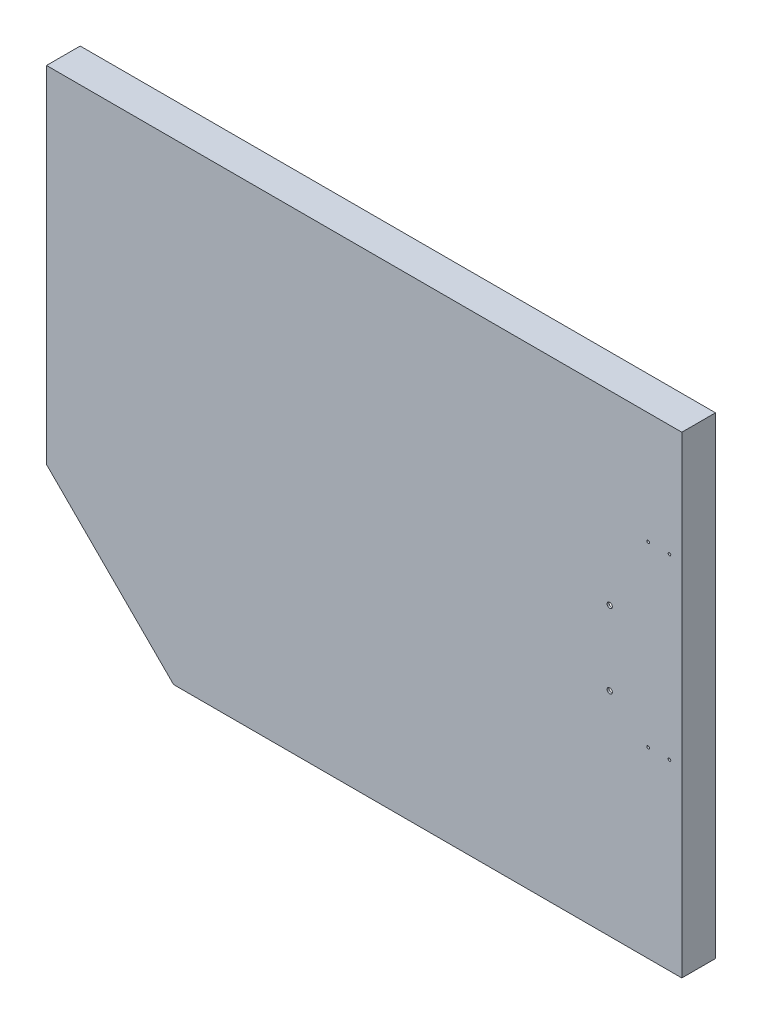
SolidWorks part; units mm, degrees
ref_plane "前视基准面" through (0, 0, 0) normal (0, 0, 1) x (1, 0, 0)
ref_plane "上视基准面" through (0, 0, 0) normal (0, 1, 0) x (1, 0, 0)
ref_plane "右视基准面" through (0, 0, 0) normal (1, 0, 0) x (0, 0, -1)
other "Configuration Table"
sketch "草图1" plane through (0, 0, 0) normal (0, 0, 1) x (1, 0, 0)
  line L0 (-300, -350) -> (500, -350)
  line L1 (-500, -150) -> (-300, -350)
  line L2 (-500, 394) -> (-500, -150)
  line L3 (500, -350) -> (500, 394)
  line L4 (500, 394) -> (-500, 394)
  dimension "D1" = 1000
  dimension "D2" = 744
  dimension "D3" = 200
  dimension "D4" = 200
  dimension "D5" = 800
  dimension "D6" = 350
  dimension "D7" = 500
extrude "拉伸-薄壁1" add sketch "草图1" along normal blind 50 thin thin type one direction reverse wall 3
sketch "草图2" plane through (0, 0, 50) normal (0, 0, 1) x (1, 0, 0)
  line L5 (-500, -150) -> (-300, -350)
  line L6 (-300, -350) -> (500, -350)
  line L7 (500, -350) -> (500, 394)
  line L8 (500, 394) -> (-500, 394)
  line L9 (-500, 394) -> (-500, -150)
  line L10 (-500, -150) -> (-300, -350)
  line L11 (-300, -350) -> (500, -350)
  line L12 (500, -350) -> (500, 394)
  line L13 (500, 394) -> (-500, 394)
  line L14 (-500, 394) -> (-500, -150)
  dimension "D1" = 0
extrude "凸台-拉伸1" add sketch "草图2" along normal blind 3
sketch "草图3" plane through (0, 0, 53) normal (0, 0, 1) x (1, 0, 0)
  circle A0 centre (386.5, 101.25) radius 4.1
  circle A1 centre (386.5, -15.25) radius 4.1
  dimension "D1" = 8.2
extrude "切除-拉伸1" cut sketch "草图3" against normal up to next
sketch "草图6" plane through (-500, 0, 0) normal (-1, 0, 0) x (0, 0, 1)
  point P0 (21, 284)
  point P3 (21, 254)
  point P6 (21, 54)
  point P9 (21, 24)
hole_wizard "M8 螺纹孔1" positions "草图6" profile "草图5" tap size "M8" standard "GB"
sketch "草图5" plane through (-500, 284, 21) normal (0, 1, 0) x (0, 0, 1)
  line L0 (0, 0) -> (0, 24.2929)
  line L1 (0, 24.2929) -> (3.4, 22.25)
  line L2 (3.4, 22.25) -> (3.4, 0)
  line L5 (3.4, 0) -> (0, 0)
  line L10 (0, 24.2929) -> (-3.4, 22.25) construction
  line L11 (0, -6.35) -> (0, 107.95) construction
  dimension "螺纹孔钻头直径" = 6.8
  dimension "螺纹孔钻头深度" = 22.25
  dimension "导头角度" = 118
cosmetic thread "孔螺纹线1" parameters "D1"=16, "D2"=8
cosmetic thread "孔螺纹线2" parameters "D1"=16, "D2"=8
cosmetic thread "孔螺纹线3" parameters "D1"=16, "D2"=8
cosmetic thread "孔螺纹线4" parameters "D1"=16, "D2"=8
sketch "草图9" plane through (0, 0, 53) normal (0, 0, 1) x (1, 0, 0)
  point P0 (447.0147, -62)
  point P3 (480.5147, -62)
  point P6 (447.0147, 218)
  point P9 (480.5147, 218)
hole_wizard "M5 螺纹孔1" positions "草图9" profile "草图8" tap size "M5" standard "GB" end condition up to next
sketch "草图8" plane through (447.0147, -62, 53) normal (1, 0, 0) x (0, -1, 0)
  line L0 (0, 0) -> (0, 3)
  line L1 (0, 3) -> (2.1, 3)
  line L2 (2.1, 3) -> (2.1, 0)
  line L5 (2.1, 0) -> (0, 0)
  line L11 (0, -6.35) -> (0, 107.95) construction
  dimension "通孔螺纹孔钻头直径" = 4.2
  dimension "通孔螺纹孔钻头深度" = 3
cosmetic thread "孔螺纹线5" parameters "D2"=5
cosmetic thread "孔螺纹线6" parameters "D2"=5
cosmetic thread "孔螺纹线7" parameters "D2"=5
cosmetic thread "孔螺纹线8" parameters "D2"=5
